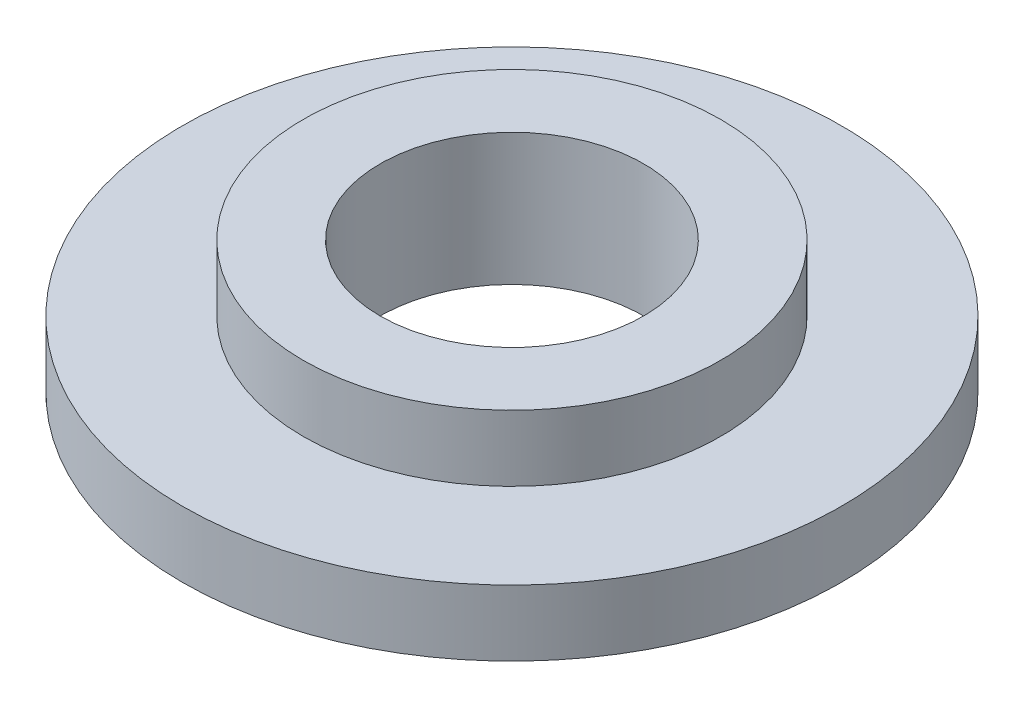
from build123d import *

# Parameters (mm, degrees)
SKETCH1_R           = 15
BOSS_EXTRUDE1_DEPTH = 3
SKETCH2_R           = 9.5
BOSS_EXTRUDE2_DEPTH = 3
SKETCH3_R           = 6
CUT_EXTRUDE1_DEPTH  = 10


with BuildPart() as part:
    # Sketch1 → Boss-Extrude1 (new body)
    with BuildSketch(Plane(origin=(0, 0, 0), x_dir=(1, 0, 0), z_dir=(0, 1, 0))):
        with Locations(Location((0, 0, 0), (0, 0, 270))):
            Circle(SKETCH1_R)
    extrude(amount=BOSS_EXTRUDE1_DEPTH)

    # Sketch2 → Boss-Extrude2 (add)
    with BuildSketch(Plane(origin=(0, 3, 0), x_dir=(1, 0, 0), z_dir=(0, 1, 0))):
        with Locations(Location((0, 0, 0), (0, 0, 270))):
            Circle(SKETCH2_R)
    extrude(amount=BOSS_EXTRUDE2_DEPTH)

    # Sketch3 → Cut-Extrude1 (cut)
    with BuildSketch(Plane(origin=(0, 6, 0), x_dir=(1, 0, 0), z_dir=(0, 1, 0))):
        with Locations(Location((0, 0, 0), (0, 0, 270))):
            Circle(SKETCH3_R)
    extrude(amount=-CUT_EXTRUDE1_DEPTH, mode=Mode.SUBTRACT)


solid = part.part
